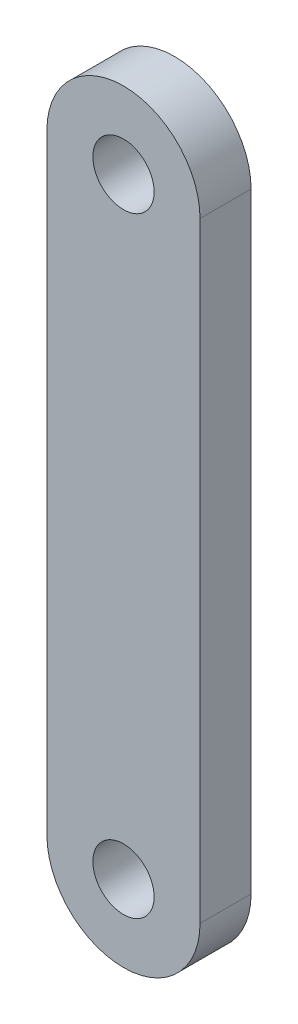
from build123d import *

# Parameters (mm, degrees)
SKETCH2_R           = 6
BOSS_EXTRUDE1_DEPTH = 10


with BuildPart() as part:
    # Sketch2 → Boss-Extrude1 (new body)
    with BuildSketch(Plane.XY.offset(-10)):
        with BuildLine():
            Line((70, 40), (70, -79.604289692))
            ThreePointArc((70, -79.604289692), (85, -94.604289692), (100, -79.604289692))
            Line((100, -79.604289692), (100, 40))
            ThreePointArc((100, 40), (85, 55), (70, 40))
        make_face()
        with Locations((85, 40)):
            Circle(SKETCH2_R, mode=Mode.SUBTRACT)
        with Locations((85, -79.604289692)):
            Circle(SKETCH2_R, mode=Mode.SUBTRACT)
    extrude(amount=BOSS_EXTRUDE1_DEPTH)


solid = part.part
